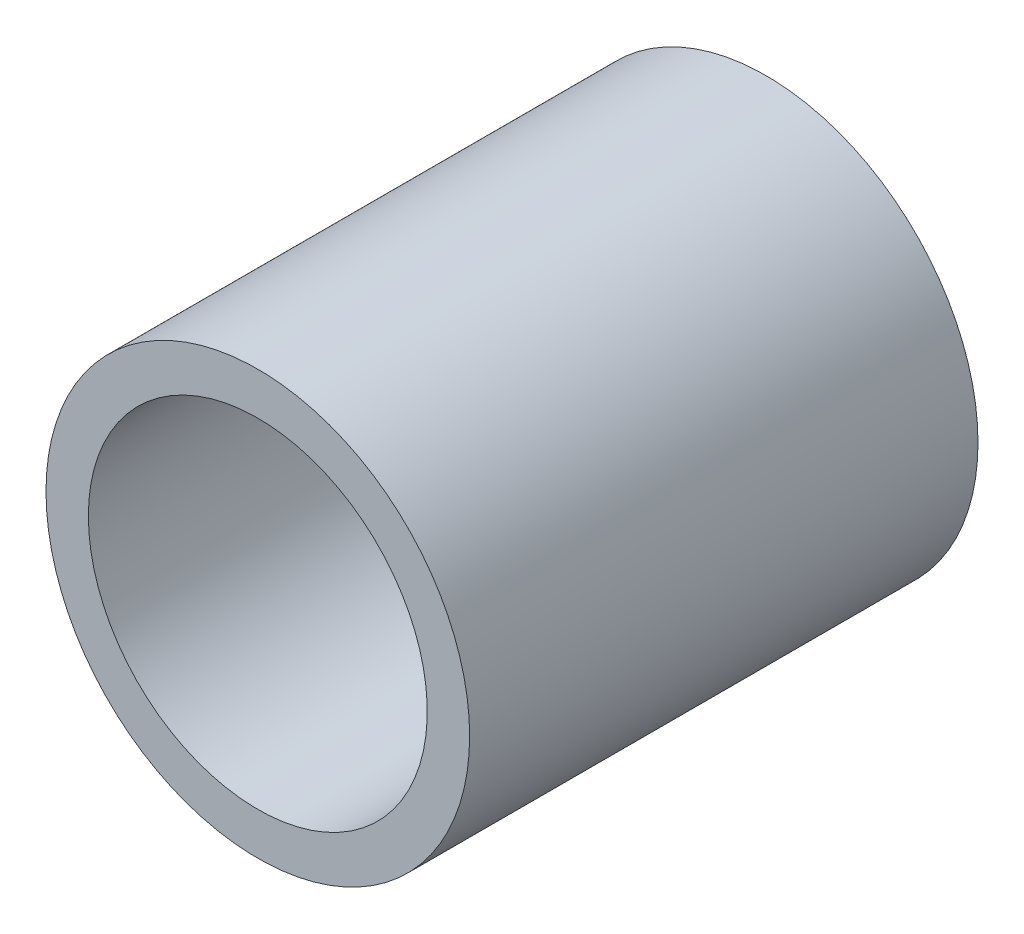
from build123d import *

# Parameters (mm, degrees)
SKETCH1_R           = 75
SKETCH1_R_2         = 60
BOSS_EXTRUDE1_DEPTH = 180


with BuildPart() as part:
    # Sketch1 → Boss-Extrude1 (new body)
    with BuildSketch(Plane.XY):
        with Locations(Location((0, 0, 0), (0, 0, 180))):
            Circle(SKETCH1_R)
        with Locations(Location((0, 0, 0), (0, 0, 180))):
            Circle(SKETCH1_R_2, mode=Mode.SUBTRACT)
    extrude(amount=BOSS_EXTRUDE1_DEPTH)


solid = part.part
